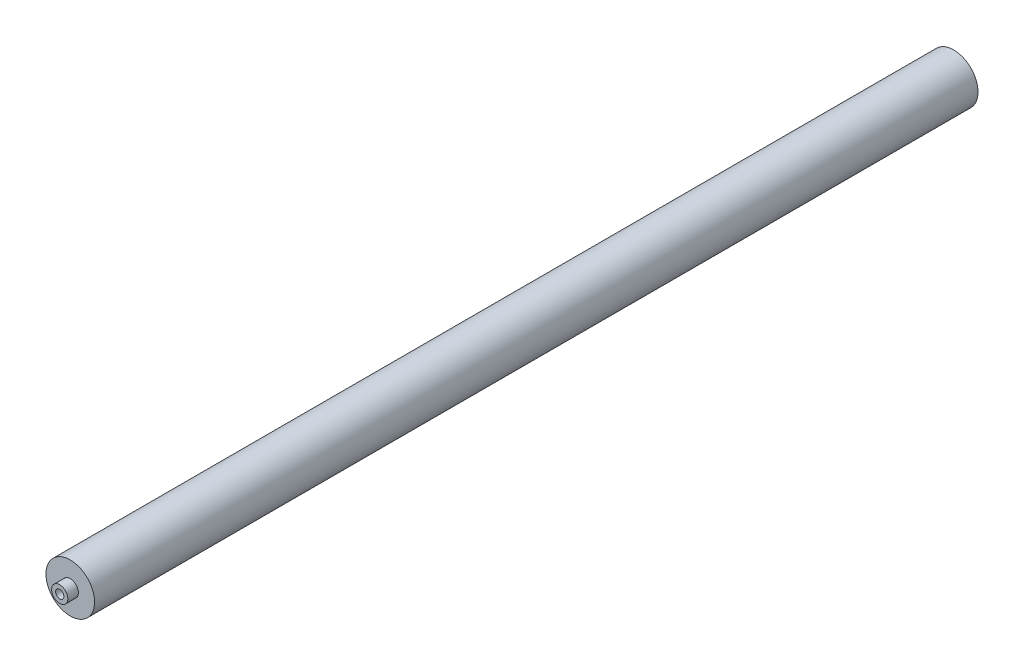
from build123d import *

# Parameters (mm, degrees)
SKETCH1_R              = 30
BOSS_EXTRUDE1_DEPTH    = 1090
SKETCH2_R              = 10
BOSS_EXTRUDE2_DEPTH    = 13
BOSS_EXTRUDE3_START    = 13
SKETCH3_R              = 10
BOSS_EXTRUDE3_DEPTH    = 13
M12_TAPPED_HOLE1_D     = 10.2
M12_TAPPED_HOLE1_DEPTH = 25.25
M12_TAPPED_HOLE1_TIP   = 3.064389157
M12_TAPPED_HOLE2_D     = 10.2
M12_TAPPED_HOLE2_DEPTH = 25.25
M12_TAPPED_HOLE2_TIP   = 3.064389157


with BuildPart() as part:
    # Sketch1 → Boss-Extrude1 (new body)
    with BuildSketch(Plane.XY):
        Circle(SKETCH1_R)
    extrude(amount=BOSS_EXTRUDE1_DEPTH)

    # Sketch2 → Boss-Extrude2 (add)
    with BuildSketch(Plane.XY.offset(1090)):
        with Locations(Location((0, 0, 0), (0, 0, 180))):
            Circle(SKETCH2_R)
    extrude(amount=BOSS_EXTRUDE2_DEPTH)

    # Sketch3 → Boss-Extrude3 (add)
    with BuildSketch(Plane(origin=(0, 0, 0), x_dir=(-1, 0, 0), z_dir=(0, 0, -1)).offset(BOSS_EXTRUDE3_START)):
        Circle(SKETCH3_R)
    extrude(amount=-BOSS_EXTRUDE3_DEPTH)

    # M12 Tapped Hole1
    with Locations(Plane(origin=(0, 0, -13), x_dir=(-1, 0, 0), z_dir=(0, 0, -1))):
        with Locations((0, 0)):
            Hole(M12_TAPPED_HOLE1_D / 2, depth=M12_TAPPED_HOLE1_DEPTH)
            with Locations((0, 0, -(M12_TAPPED_HOLE1_DEPTH + M12_TAPPED_HOLE1_TIP / 2))):  # 118° drill point
                Cone(0, M12_TAPPED_HOLE1_D / 2, M12_TAPPED_HOLE1_TIP, mode=Mode.SUBTRACT)

    # M12 Tapped Hole2
    with Locations(Plane.XY.offset(1103)):
        with Locations((0, 0)):
            Hole(M12_TAPPED_HOLE2_D / 2, depth=M12_TAPPED_HOLE2_DEPTH)
            with Locations((0, 0, -(M12_TAPPED_HOLE2_DEPTH + M12_TAPPED_HOLE2_TIP / 2))):  # 118° drill point
                Cone(0, M12_TAPPED_HOLE2_D / 2, M12_TAPPED_HOLE2_TIP, mode=Mode.SUBTRACT)


solid = part.part
